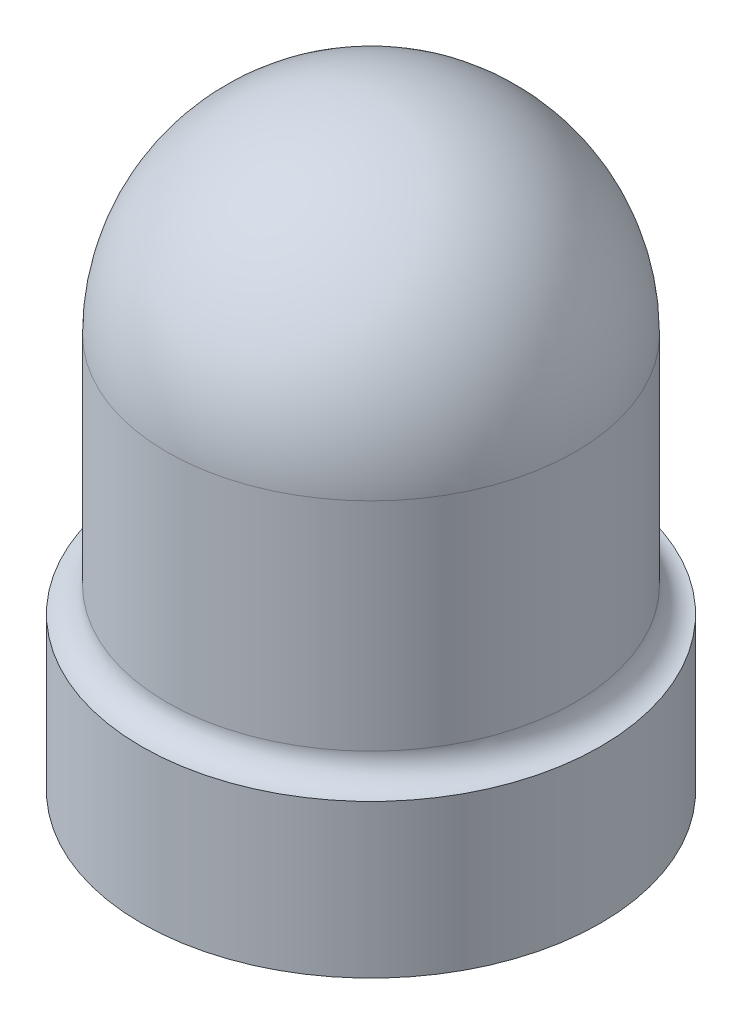
from build123d import *

# Parameters (mm, degrees)
SKETCH3_R          = 2.5
CUT_EXTRUDE1_DEPTH = 40
CHAMFER1_SIZE      = 1.5


with BuildPart() as part:
    # Sketch2 → Revolve1 (revolve)
    with BuildSketch(Plane.XY, mode=Mode.PRIVATE) as revolve1_sk:
        with BuildLine():
            Line((-16, 31), (-16, 14))
            ThreePointArc((-16, 14), (-16.585786438, 12.585786438), (-18, 12))
            Line((-18, 12), (-18, 0))
            Line((-18, 0), (-13, 0))
            Line((-13, 0), (-13, 15))
            Line((-13, 15), (-12, 15))
            Line((-12, 15), (-12, 31))
            ThreePointArc((-12, 31), (-8.485281374, 39.485281374), (0, 43))
            Line((0, 43), (0, 47))
            ThreePointArc((0, 47), (-11.313708499, 42.313708499), (-16, 31))
        make_face()
    revolve(revolve1_sk.sketch.rotate(Axis((0, -51.943033939, 0), (0, 1, 0)), 180), axis=Axis((0, -51.943033939, 0), (0, 1, 0)))

    # Sketch3 → Cut-Extrude1 (cut)
    with BuildSketch(Plane(origin=(0, 0, 0), x_dir=(0, 0, -1), z_dir=(1, 0, 0))):
        with Locations((0, 6)):
            Circle(SKETCH3_R)
    extrude(amount=-CUT_EXTRUDE1_DEPTH, mode=Mode.SUBTRACT)

    # Chamfer1
    chamfer1_edges = [part.edges().sort_by_distance(p)[0] for p in [
        (-13, 0, 0),
    ]]
    chamfer(chamfer1_edges, length=CHAMFER1_SIZE)


solid = part.part
